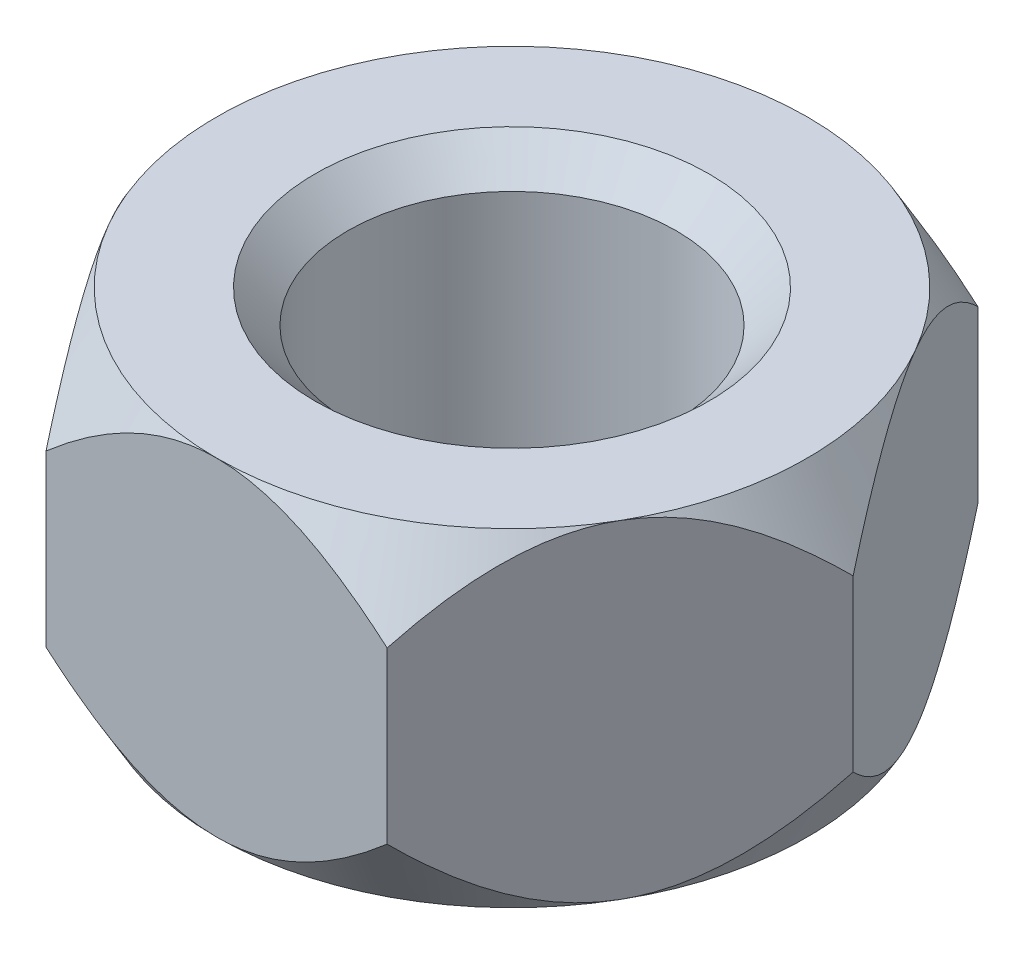
SolidWorks part; units mm, degrees
ref_plane "Front Plane" through (0, 0, 0) normal (0, 0, 1) x (1, 0, 0)
ref_plane "Top Plane" through (0, 0, 0) normal (0, 1, 0) x (1, 0, 0)
ref_plane "Right Plane" through (0, 0, 0) normal (1, 0, 0) x (0, 0, -1)
sketch "Sketch1" plane through (0, 0, 0) normal (0, 1, 0) x (1, 0, 0)
  line L1 (2.5981, 4.5) -> (-2.5981, 4.5)
  line L2 (-2.5981, 4.5) -> (-5.1962, 0)
  line L3 (-5.1962, 0) -> (-2.5981, -4.5)
  line L4 (-2.5981, -4.5) -> (2.5981, -4.5)
  line L5 (2.5981, -4.5) -> (5.1962, 0)
  line L6 (5.1962, 0) -> (2.5981, 4.5)
  circle A0 centre (0, 0) radius 4.5 construction
  dimension "D1" = 9
extrude "Boss-Extrude1" add sketch "Sketch1" along normal blind 5
sketch "Sketch2" plane through (0, 5, 0) normal (0, 1, 0) x (1, 0, 0)
  circle A0 centre (0, 0) radius 2.5
  dimension "D1" = 5
extrude "Cut-Extrude1" cut sketch "Sketch2" against normal blind 5
cosmetic thread "Cosmetic Thread1" parameters "D1"=5, "D2"=6
sketch "Sketch3" plane through (0, 5, 0) normal (0, 1, 0) x (1, 0, 0)
  circle A0 centre (0, 0) radius 4.5
  dimension "D1" = 9
extrude "Cut-Extrude2" cut sketch "Sketch3" against normal blind 5 draft 30 flip side to cut
sketch "Sketch4" plane through (0, 0, 0) normal (0, -1, 0) x (1, 0, 0)
  circle A0 centre (0, 0) radius 4.5
extrude "Cut-Extrude3" cut sketch "Sketch4" against normal blind 5 draft 30 flip side to cut
chamfer "Chamfer1" distance 0.5 angle 45 1 edges at (0, 5, 2.5)
chamfer "Chamfer2" distance 0.5 angle 45 1 edges at (0, 0, 2.5)
